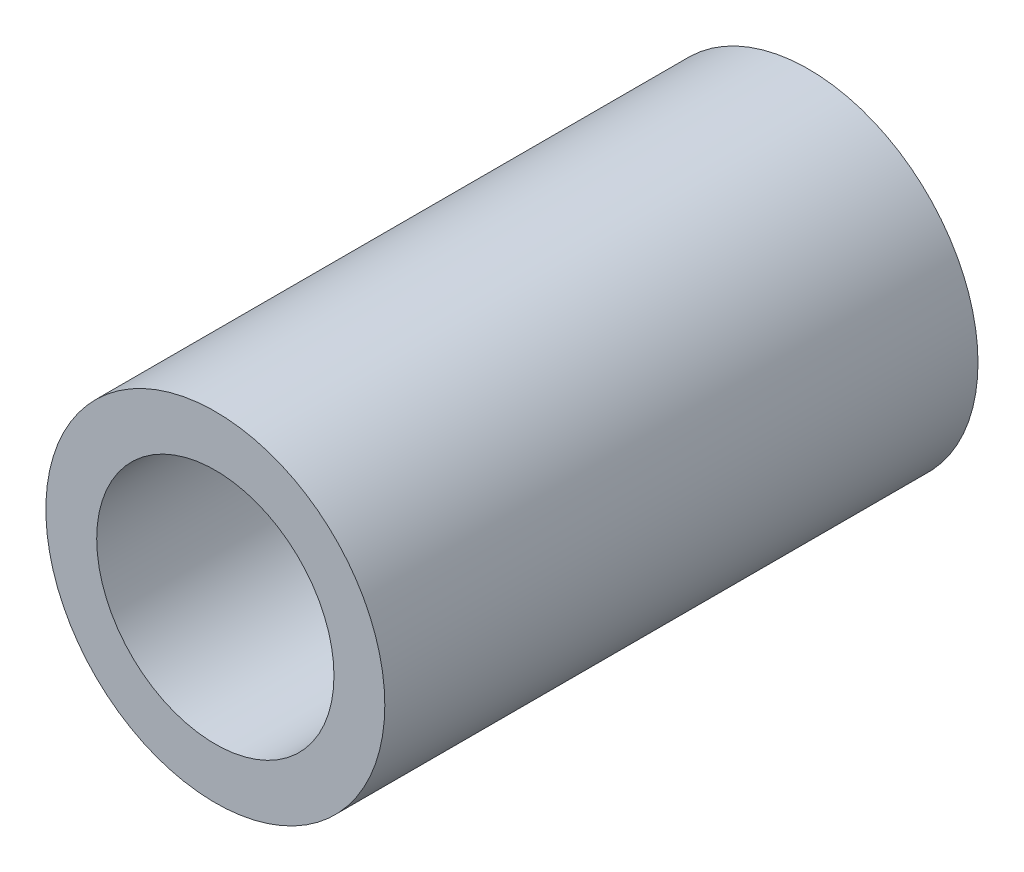
from build123d import *

# Parameters (mm, degrees)
SKETCH1_R           = 10
SKETCH1_R_2         = 7
BOSS_EXTRUDE1_DEPTH = 35


with BuildPart() as part:
    # Sketch1 → Boss-Extrude1 (new body)
    with BuildSketch(Plane.XY):
        Circle(SKETCH1_R)
        Circle(SKETCH1_R_2, mode=Mode.SUBTRACT)
    extrude(amount=BOSS_EXTRUDE1_DEPTH)


solid = part.part
